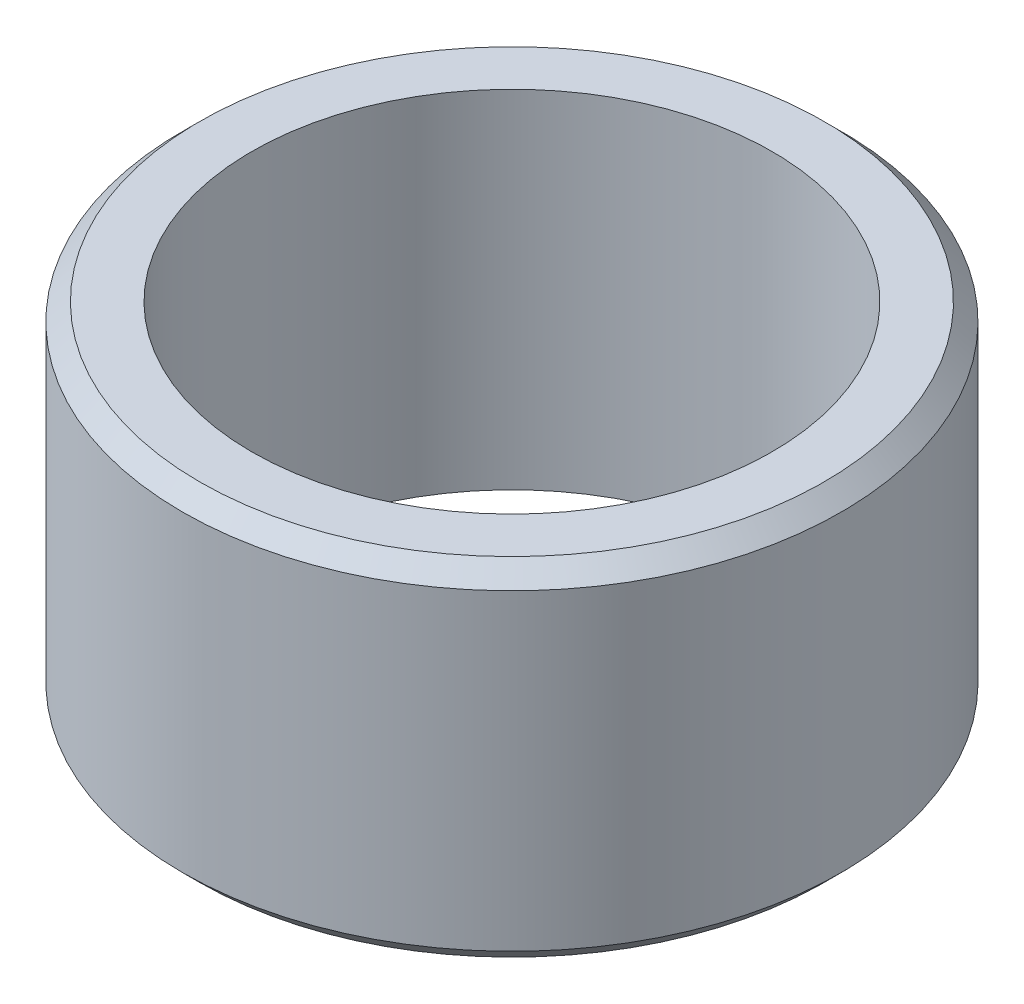
from build123d import *

# Parameters (mm, degrees)
SKETCH1_R           = 19
SKETCH1_R_2         = 15
BOSS_EXTRUDE1_DEPTH = 20
CHAMFER1_SIZE       = 1


with BuildPart() as part:
    # Sketch1 → Boss-Extrude1 (new body)
    with BuildSketch(Plane(origin=(0, 0, 0), x_dir=(1, 0, 0), z_dir=(0, 1, 0))):
        with Locations(Location((0, 0, 0), (0, 0, 270))):
            Circle(SKETCH1_R)
        with Locations(Location((0, 0, 0), (0, 0, 270))):
            Circle(SKETCH1_R_2, mode=Mode.SUBTRACT)
    extrude(amount=BOSS_EXTRUDE1_DEPTH)

    # Chamfer1
    chamfer1_edges = [part.edges().sort_by_distance(p)[0] for p in [
        (0, 0, -19),
        (0, 20, -19),
    ]]
    chamfer(chamfer1_edges, length=CHAMFER1_SIZE)


solid = part.part
